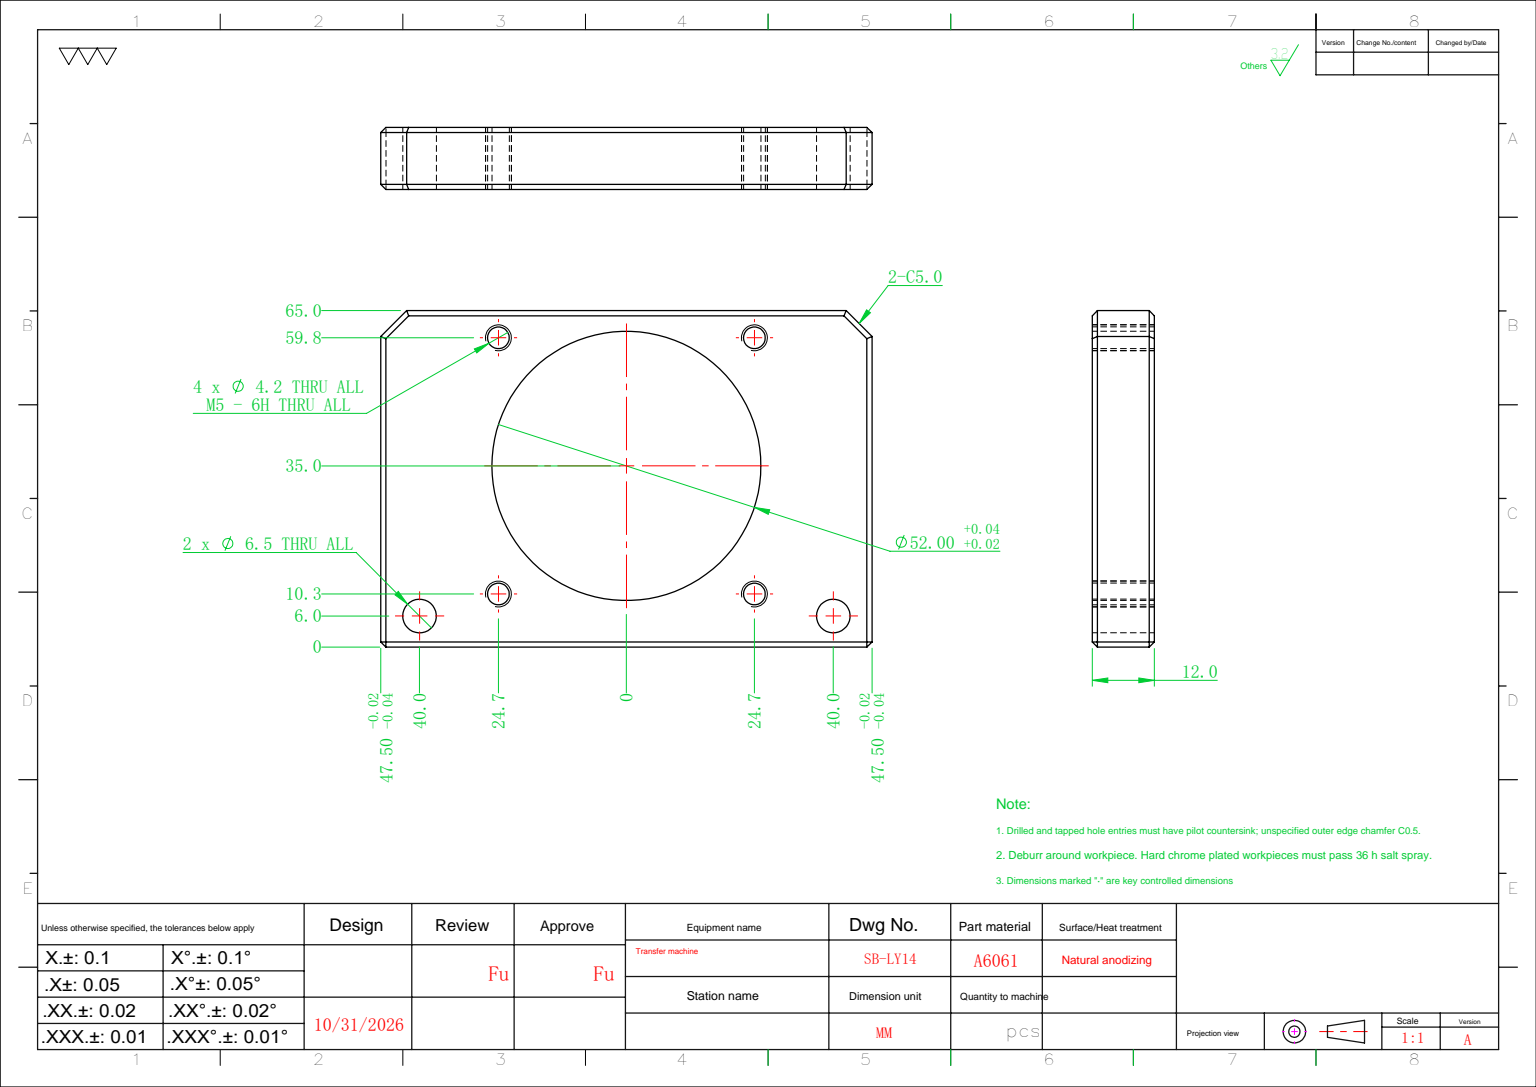
SolidWorks part; units mm, degrees
ref_plane "前视基准面" through (0, 0, 0) normal (0, 0, 1) x (1, 0, 0)
ref_plane "上视基准面" through (0, 0, 0) normal (0, 1, 0) x (1, 0, 0)
ref_plane "右视基准面" through (0, 0, 0) normal (1, 0, 0) x (0, 0, -1)
sketch "草图1" plane through (0, 0, 0) normal (0, 0, 1) x (1, 0, 0)
  line L1 (-47.5, -32.5) -> (47.5, -32.5)
  line L2 (-47.5, -32.5) -> (-47.5, 32.5)
  line L3 (-47.5, 32.5) -> (47.5, 32.5)
  line L4 (47.5, -32.5) -> (47.5, 32.5)
  line L5 (-47.5, -32.5) -> (47.5, 32.5) construction
  line L6 (-47.5, 32.5) -> (47.5, -32.5) construction
  point P0 (0, 0)
  dimension "D1" = 95
  dimension "D2" = 65
extrude "凸台-拉伸1" add sketch "草图1" along normal blind 12
hole_wizard "Ø6.5 (6.5) 直径孔1" positions "草图2" profile "草图3" hole size "Ø6.5" standard "ISO" end condition through all
sketch "草图2" plane through (0, 0, 12) normal (0, 0, 1) x (1, 0, 0)
  line L0 (0, 0) -> (0, -55.2693) construction
  line L2 (-47.5, -32.5) -> (47.5, -32.5) construction
  point P0 (-40, -26.5)
  point P8 (40, -26.5)
  dimension "D1" = 80
  dimension "D2" = 6
sketch "草图3" plane through (-40, -26.5, 12) normal (1, 0, 0) x (0, -1, 0)
  line L0 (0, 0) -> (0, 12)
  line L1 (0, 12) -> (3.25, 12)
  line L2 (3.25, 12) -> (3.25, 0)
  line L5 (3.25, 0) -> (0, 0)
  line L11 (0, -6.35) -> (0, 107.95) construction
  dimension "通孔孔直径" = 6.5
  dimension "通孔孔深度" = 12
chamfer "倒角1" distance 5 angle 45 2 edges at (47.5, 32.5, 6) (-47.5, 32.5, 6)
sketch "草图4" plane through (0, 0, 0) normal (0, 0, -1) x (-1, 0, 0)
  line L0 (0, 0) -> (0, 39.3446) construction
  line L1 (47.5, -32.5) -> (-47.5, -32.5) construction
  circle A0 centre (0, 2.5) radius 26
  dimension "D1" = 52
  dimension "D2" = 35
extrude "切除-拉伸1" cut sketch "草图4" against normal through all
hole_wizard "M5 螺纹孔1" positions "草图5" profile "草图6" tap size "M5" standard "ISO" end condition through all
sketch "草图5" plane through (0, 0, 12) normal (0, 0, 1) x (1, 0, 0)
  line L0 (0, 2.5) -> (-53.4101, 2.5) construction
  line L2 (0, 2.5) -> (0, -36.2578) construction
  point P0 (-24.7487, 27.25)
  point P3 (24.7487, 27.25)
  point P6 (24.7487, -22.25)
  point P9 (-24.7487, -22.25)
  dimension "D1" = 49.4975
  dimension "D2" = 49.5
sketch "草图6" plane through (-24.7487, 27.25, 12) normal (1, 0, 0) x (0, -1, 0)
  line L0 (0, 0) -> (0, 12)
  line L1 (0, 12) -> (2.1, 12)
  line L2 (2.1, 12) -> (2.1, 0)
  line L5 (2.1, 0) -> (0, 0)
  line L11 (0, -6.35) -> (0, 107.95) construction
  dimension "通孔螺纹孔钻头直径" = 4.2
  dimension "通孔螺纹孔钻头深度" = 12
cosmetic thread "孔螺蚊线1" parameters "D2"=5
cosmetic thread "孔螺蚊线2" parameters "D2"=5
cosmetic thread "孔螺蚊线3" parameters "D2"=5
cosmetic thread "孔螺蚊线4" parameters "D2"=5
chamfer "倒角2" distance 1 angle 45 14 edges at (-47.5, -32.5, 6) (0, -32.5, 12) (-47.5, -2.5, 12) (-45, 30, 12) (0, 32.5, 12) (45, 30, 12) (47.5, -2.5, 12) (47.5, -32.5, 6) (-45, 30, 0) (-47.5, -2.5, 0) (0, -32.5, 0) (47.5, -2.5, 0) (45, 30, 0) (0, 32.5, 0)
